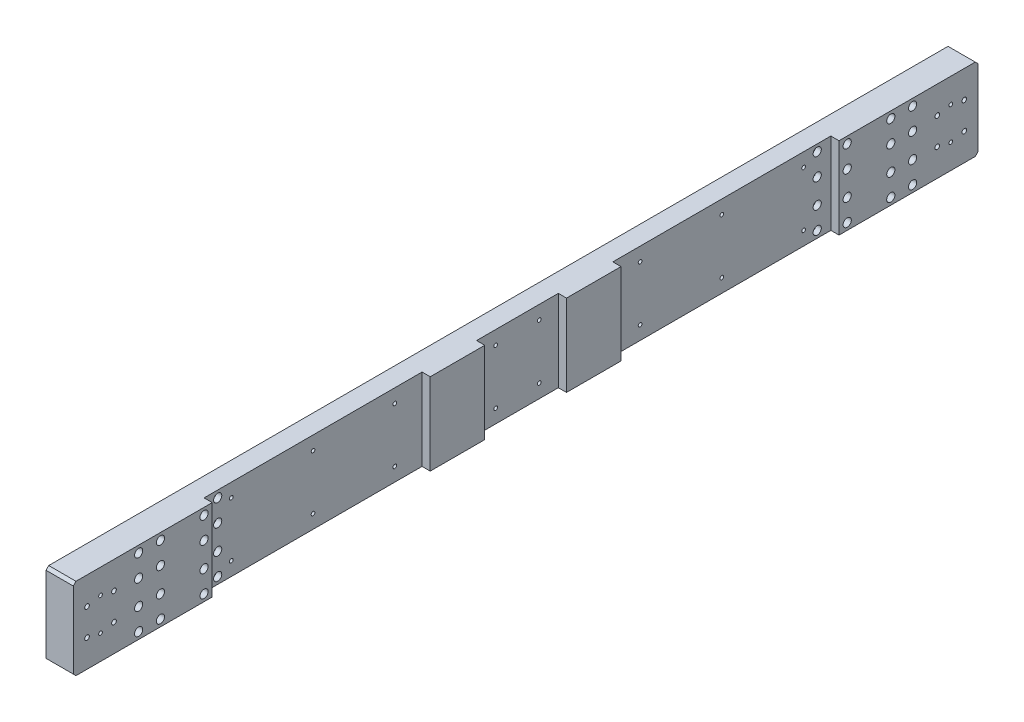
SolidWorks part; units mm, degrees
ref_plane "前视基准面" through (0, 0, 0) normal (0, 0, 1) x (1, 0, 0)
ref_plane "上视基准面" through (0, 0, 0) normal (0, 1, 0) x (1, 0, 0)
ref_plane "右视基准面" through (0, 0, 0) normal (1, 0, 0) x (0, 0, -1)
sketch "草图1" plane through (0, 0, 0) normal (1, 0, 0) x (0, 0, -1)
  line L1 (-830, 75) -> (830, 75)
  line L2 (-830, 75) -> (-830, -75)
  line L3 (-830, -75) -> (830, -75)
  line L4 (830, 75) -> (830, -75)
  line L5 (-830, 75) -> (830, -75) construction
  line L6 (-830, -75) -> (830, 75) construction
  point P0 (0, 0)
  dimension "D1" = 1660
  dimension "D2" = 150
extrude "凸台-拉伸1" add sketch "草图1" along normal blind 50
hole_wizard "M10 螺纹孔1" positions "草图2" profile "草图3" tap size "M10" standard "ISO" end condition through all
sketch "草图2" plane through (50, 0, 0) normal (1, 0, 0) x (0, 0, -1)
  line L0 (-830, 0) -> (-584.7864, 0) construction
  line L1 (-830, 75) -> (-830, -75) construction
  line L3 (-780, 0) -> (-780, 100.8421) construction
  line L5 (-804.7487, 24.7487) -> (-780, 0) construction
  circle A0 centre (-780, 0) radius 35 construction
  point P0 (-804.7487, 24.7487)
  point P2 (-755.2513, 24.7487)
  point P4 (-804.7487, -24.7487)
  point P6 (-755.2513, -24.7487)
  dimension "D2" = 70
  dimension "D1" = 45
  dimension "D3" = 780
sketch "草图3" plane through (50, 24.7487, 804.7487) normal (0, 1, 0) x (0, 0, -1)
  line L0 (0, 0) -> (0, 50)
  line L1 (0, 50) -> (4.25, 50)
  line L2 (4.25, 50) -> (4.25, 0)
  line L5 (4.25, 0) -> (0, 0)
  line L11 (0, -6.35) -> (0, 107.95) construction
  dimension "通孔螺纹孔钻头直径" = 8.5
  dimension "通孔螺纹孔钻头深度" = 50
cosmetic thread "孔螺蚊线1" parameters "D2"=10
cosmetic thread "孔螺蚊线2" parameters "D2"=10
cosmetic thread "孔螺蚊线3" parameters "D2"=10
cosmetic thread "孔螺蚊线4" parameters "D2"=10
mirror "镜向1" about plane through (0, 0, 0) normal (0, 0, 1) of "M10 螺纹孔1"
sketch "草图4" plane through (50, 0, 0) normal (1, 0, 0) x (0, 0, -1)
  line L0 (0, 0) -> (0, 173.6925) construction
  line L1 (-75, 75) -> (75, 75)
  line L2 (-75, 75) -> (-75, -75)
  line L3 (-75, -75) -> (75, -75)
  line L4 (75, 75) -> (75, -75)
  line L5 (-75, 75) -> (75, -75) construction
  line L6 (-75, -75) -> (75, 75) construction
  line L7 (-575, 75) -> (-175, 75)
  line L8 (-575, 75) -> (-575, -75)
  line L9 (-575, -75) -> (-175, -75)
  line L10 (-175, 75) -> (-175, -75)
  line L11 (-575, 75) -> (-175, -75) construction
  line L12 (-575, -75) -> (-175, 75) construction
  line L13 (175, 75) -> (575, 75)
  line L14 (175, 75) -> (175, -75)
  line L15 (175, -75) -> (575, -75)
  line L16 (575, 75) -> (575, -75)
  line L17 (175, 75) -> (575, -75) construction
  line L18 (175, -75) -> (575, 75) construction
  line L19 (830, 75) -> (-830, 75) construction
  point P0 (0, 0)
  point P6 (-375, 0)
  point P11 (375, 0)
  dimension "D1" = 150
  dimension "D2" = 400
  dimension "D3" = 100
extrude "切除-拉伸1" cut sketch "草图4" against normal blind 15
hole_wizard "M8 螺纹孔1" positions "草图5" profile "草图6" tap size "M8" standard "GB" end condition through all
sketch "草图5" plane through (35, 0, 0) normal (1, 0, 0) x (0, 0, -1)
  line L0 (-375, -75) -> (-375, 137.5663) construction
  line L1 (-575, -75) -> (-175, -75) construction
  line L3 (-575, 0) -> (-251.3676, 0) construction
  line L4 (-575, 75) -> (-575, -75) construction
  point P0 (-525, 50)
  point P2 (-375, 50)
  point P4 (-225, 50)
  point P6 (-525, -50)
  point P8 (-375, -50)
  point P10 (-225, -50)
  dimension "D1" = 300
  dimension "D2" = 100
sketch "草图6" plane through (35, 50, 525) normal (0, 1, 0) x (0, 0, -1)
  line L0 (0, 0) -> (0, 35)
  line L1 (0, 35) -> (3.4, 35)
  line L2 (3.4, 35) -> (3.4, 0)
  line L5 (3.4, 0) -> (0, 0)
  line L11 (0, -6.35) -> (0, 107.95) construction
  dimension "通孔螺纹孔钻头直径" = 6.8
  dimension "通孔螺纹孔钻头深度" = 35
cosmetic thread "孔螺蚊线15" parameters "D1"=25, "D2"=8
cosmetic thread "孔螺蚊线16" parameters "D1"=25, "D2"=8
cosmetic thread "孔螺蚊线17" parameters "D1"=25, "D2"=8
cosmetic thread "孔螺蚊线18" parameters "D1"=25, "D2"=8
cosmetic thread "孔螺蚊线19" parameters "D1"=25, "D2"=8
cosmetic thread "孔螺蚊线20" parameters "D1"=25, "D2"=8
mirror "镜向2" about plane through (0, 0, 0) normal (0, 0, 1) of "M8 螺纹孔1"
hole_wizard "M8 螺纹孔2" positions "草图7" profile "草图8" tap size "M8" standard "GB" end condition through all
sketch "草图7" plane through (35, 0, 0) normal (1, 0, 0) x (0, 0, -1)
  line L0 (0, 145.4572) -> (0, 0) construction
  line L1 (0, 0) -> (112.5288, 0) construction
  point P0 (-40, 50)
  point P2 (40, 50)
  point P4 (-40, -50)
  point P6 (40, -50)
  dimension "D1" = 80
  dimension "D2" = 100
sketch "草图8" plane through (35, 50, 40) normal (0, 1, 0) x (0, 0, -1)
  line L0 (0, 0) -> (0, 35)
  line L1 (0, 35) -> (3.4, 35)
  line L2 (3.4, 35) -> (3.4, 0)
  line L5 (3.4, 0) -> (0, 0)
  line L11 (0, -6.35) -> (0, 107.95) construction
  dimension "通孔螺纹孔钻头直径" = 6.8
  dimension "通孔螺纹孔钻头深度" = 35
cosmetic thread "孔螺蚊线11" parameters "D2"=8
cosmetic thread "孔螺蚊线12" parameters "D2"=8
cosmetic thread "孔螺蚊线13" parameters "D2"=8
cosmetic thread "孔螺蚊线14" parameters "D2"=8
hole_wizard "打孔尺寸(%根据)内六角圆柱头螺钉的类型1" positions "草图9" profile "草图10" counterbore size "M8" standard "GB" end condition through all
sketch "草图9" plane through (50, 0, 0) normal (1, 0, 0) x (0, 0, -1)
  line L0 (-830, 0) -> (-772.1222, 0) construction
  line L1 (-830, 75) -> (-830, -75) construction
  point P0 (-710, -22.5)
  point P2 (-710, -62.5)
  point P4 (-670, -22.5)
  point P6 (-670, -62.5)
  point P21 (-670, 62.5)
  point P22 (-670, 22.5)
  point P23 (-710, 62.5)
  point P24 (-710, 22.5)
  dimension "D1" = 40
  dimension "D2" = 45
  dimension "D3" = 40
  dimension "D4" = 120
sketch "草图10" plane through (50, -22.5, 710) normal (0, 1, 0) x (0, 0, -1)
  line L0 (0, 0) -> (0, 50)
  line L1 (0, 50) -> (4.5, 50)
  line L3 (4.5, 50) -> (4.5, 25)
  line L4 (4.5, 25) -> (7.5, 25)
  line L5 (7.5, 25) -> (7.5, 0)
  line L7 (7.5, 0) -> (0, 0)
  line L11 (0, -6.35) -> (0, 107.95) construction
  dimension "通孔孔直径" = 9
  dimension "通孔孔深度" = 50
  dimension "柱形沉头孔直径" = 15
  dimension "柱形沉头孔深度" = 25
pattern_linear "阵列(线性)1" count 2 spacing 120 along (0, 0, -1) of "打孔尺寸(%根据)内六角圆柱头螺钉的类型1"
mirror "镜向3" about plane through (0, 0, 0) normal (0, 0, 1) of "阵列(线性)1", "打孔尺寸(%根据)内六角圆柱头螺钉的类型1"
hole_wizard "M8 螺纹孔3" positions "草图12" profile "草图13" tap size "M8" standard "GB" end condition through all
sketch "草图12" plane through (50, 0, 0) normal (1, 0, 0) x (0, 0, -1)
  line L0 (-830, 0) -> (-631.8369, 0) construction
  line L1 (-830, 75) -> (-830, -75) construction
  point P0 (-780, 30)
  point P4 (-780, -30)
  dimension "D1" = 60
  dimension "D3" = 50
sketch "草图13" plane through (50, 30, 780) normal (0, 1, 0) x (0, 0, -1)
  line L0 (0, 0) -> (0, 50)
  line L1 (0, 50) -> (3.4, 50)
  line L2 (3.4, 50) -> (3.4, 0)
  line L5 (3.4, 0) -> (0, 0)
  line L11 (0, -6.35) -> (0, 107.95) construction
  dimension "通孔螺纹孔钻头直径" = 6.8
  dimension "通孔螺纹孔钻头深度" = 50
cosmetic thread "孔螺蚊线22" parameters "D2"=8
cosmetic thread "孔螺蚊线24" parameters "D2"=8
mirror "镜向4" about plane through (0, 0, 0) normal (0, 0, 1) of "M8 螺纹孔3"
chamfer "倒角1" distance 5 angle 45 4 edges at (25, -75, -830) (25, 75, -830) (25, -75, 830) (25, 75, 830)
